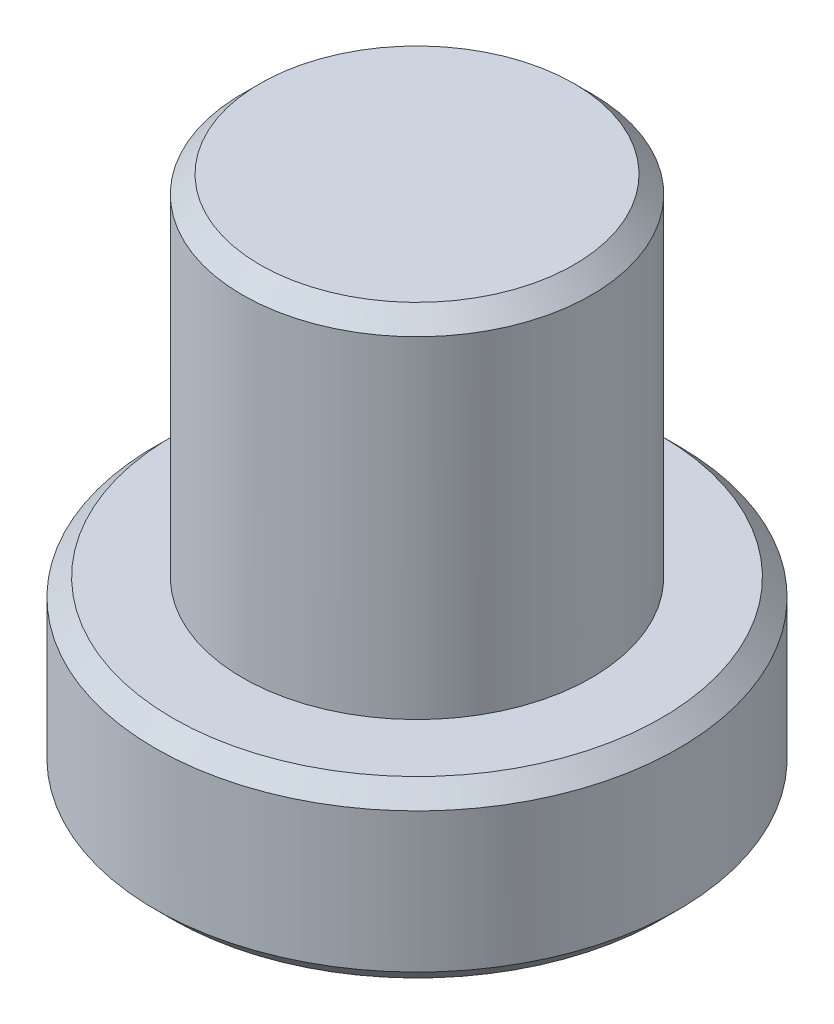
from build123d import *

# Parameters (mm, degrees)
CHAMFER1_SIZE = 0.5


with BuildPart() as part:
    # Sketch1 → Revolve1 (revolve)
    with BuildSketch(Plane(origin=(0, 0, 0), x_dir=(0, 0, -1), z_dir=(1, 0, 0))):
        Polygon((0, 15), (5, 15), (5, 5), (7.5, 5), (7.5, 0), (0, 0), align=None)
    revolve(axis=Axis((0, 0, 0), (0, 1, 0)))

    # Chamfer1
    chamfer1_edges = [part.edges().sort_by_distance(p)[0] for p in [
        (0, 0, 7.5),
        (0, 5, 7.5),
        (0, 15, 5),
    ]]
    chamfer(chamfer1_edges, length=CHAMFER1_SIZE)


solid = part.part
